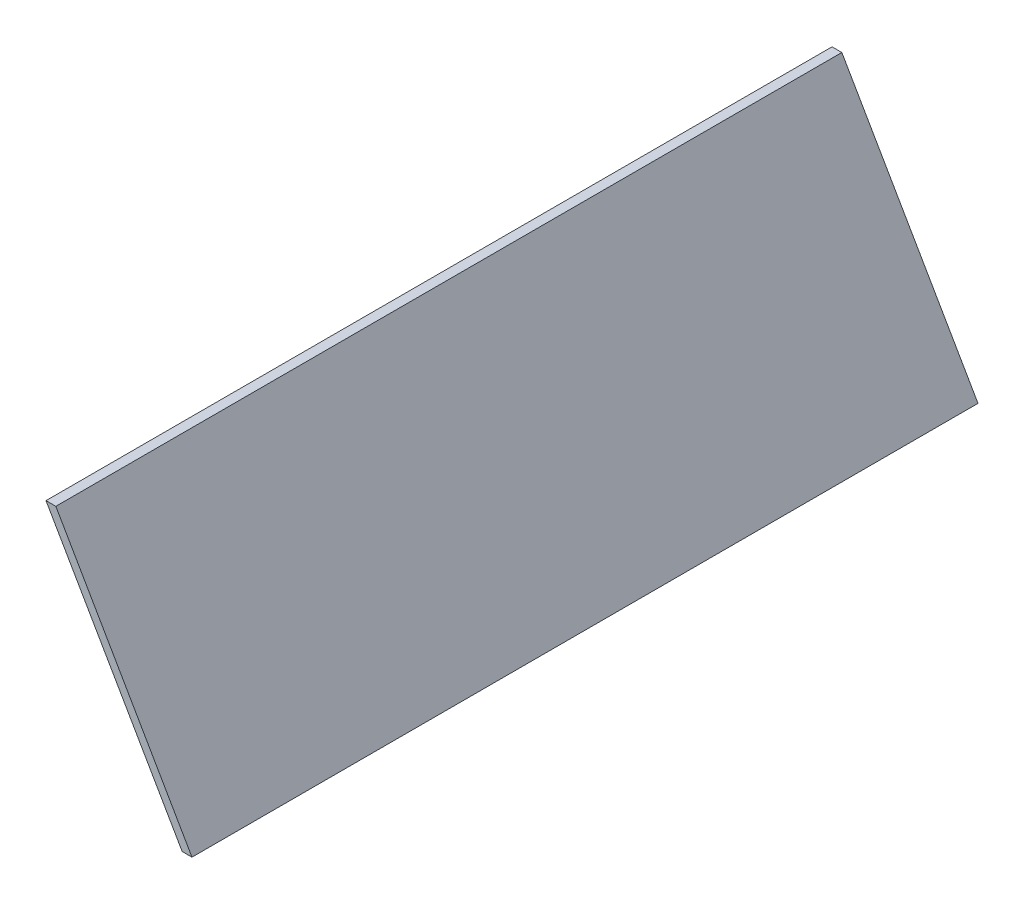
from build123d import *

# Parameters (mm, degrees)
EXTRUDE_1_DEPTH = 400


with BuildPart() as part:
    # 草图1 → 凸台-拉伸1 (new body)
    with BuildSketch(Plane.XY):
        Polygon((0, 0), (5, 0), (74.282032303, -120), (69.282032303, -120), align=None)
    extrude(amount=EXTRUDE_1_DEPTH)


solid = part.part
